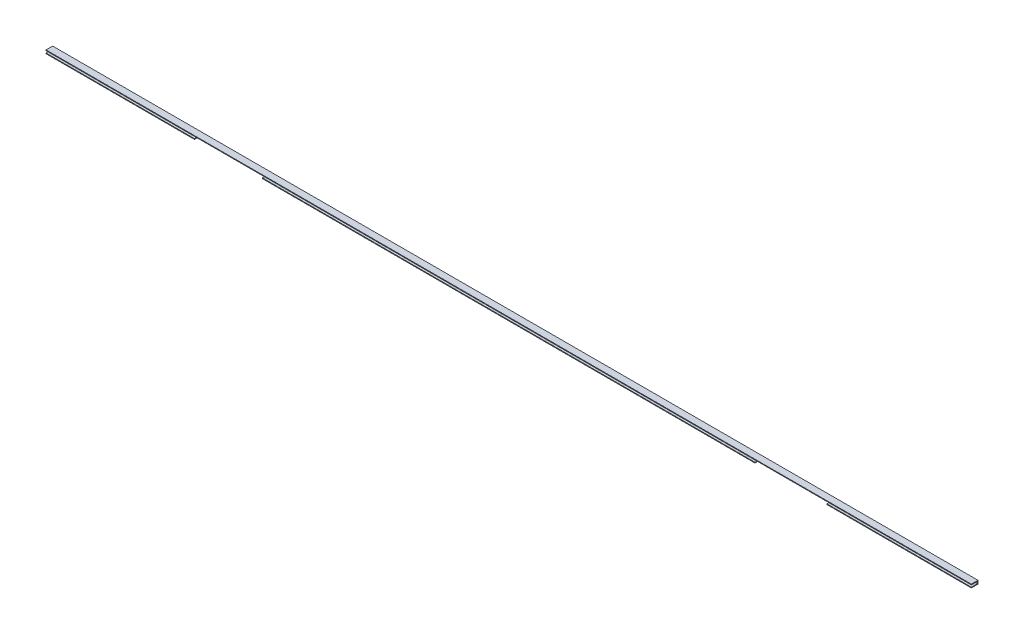
SolidWorks part; units mm, degrees
material "硅橡胶"
ref_plane "前视基准面" through (0, 0, 0) normal (0, 0, 1) x (1, 0, 0)
ref_plane "上视基准面" through (0, 0, 0) normal (0, 1, 0) x (1, 0, 0)
ref_plane "右视基准面" through (0, 0, 0) normal (1, 0, 0) x (0, 0, -1)
other "Configuration Table"
sketch "草图1" plane through (0, 0, 0) normal (0, 0, 1) x (1, 0, 0)
  line L1 (-695, -2.5) -> (695, -2.5)
  line L2 (-695, -2.5) -> (-695, 2.5)
  line L3 (-695, 2.5) -> (695, 2.5)
  line L4 (695, -2.5) -> (695, 2.5)
  line L5 (-695, -2.5) -> (695, 2.5) construction
  line L6 (-695, 2.5) -> (695, -2.5) construction
  point P0 (0, 0)
  dimension "D1" = 1390
  dimension "D2" = 5
extrude "拉伸-薄壁1" add sketch "草图1" along normal blind 10 thin thin type one direction reverse wall 1
sketch "草图2" plane through (-695, 0, 0) normal (-1, 0, 0) x (0, 0, 1)
  line L0 (10, -2.5) -> (0, -2.5) construction
  line L1 (0, 2.5) -> (1, 2.5)
  line L2 (0, 2.5) -> (0, -2.5)
  line L3 (0, -2.5) -> (1, -2.5)
  line L4 (1, 2.5) -> (1, -2.5)
  dimension "D1" = 1
extrude "凸台-拉伸1" add sketch "草图2" against normal up to surface (1389 mm away) contours L4 L3 L2 L1 up to face at (694, 0, 5)
sketch "草图3" plane through (694, 0, 0) normal (-1, 0, 0) x (0, 0, 1)
  line L4 (10, 1.5) -> (1, 1.5)
  line L5 (1, 1.5) -> (1, -1.5)
  line L6 (1, -1.5) -> (10, -1.5)
  line L7 (10, -1.5) -> (10, 1.5)
  line L8 (10, 1.5) -> (1, 1.5)
  line L9 (1, 1.5) -> (1, -1.5)
  line L10 (1, -1.5) -> (10, -1.5)
  line L11 (10, -1.5) -> (10, 1.5)
  dimension "D1" = 0
extrude "切除-拉伸1" cut sketch "草图3" against normal through all both and the other way through all
sketch "草图4" plane through (-695, 0, 0) normal (-1, 0, 0) x (0, 0, 1)
  line L1 (0, -2.5) -> (10, -2.5)
  line L2 (0, -2.5) -> (0, -1.5)
  line L3 (0, -1.5) -> (10, -1.5)
  line L4 (10, -2.5) -> (10, -1.5)
extrude "切除-拉伸2" cut sketch "草图4" along normal blind 102 from offset 325 offset against normal yes
mirror "镜向1" about plane through (0, 0, 0) normal (1, 0, 0) of "切除-拉伸2"
sketch "草图5" plane through (0, -2.5, 0) normal (0, -1, 0) x (1, 0, 0)
  line L0 (472, 10) -> (695, 10) construction
  line L1 (472, 1) -> (478, 1)
  line L2 (472, 1) -> (472, 10)
  line L3 (472, 10) -> (478, 10)
  line L4 (478, 1) -> (478, 10)
  line L6 (472, 1) -> (370, 1) construction
  dimension "D1" = 6
extrude "切除-拉伸5" cut sketch "草图5" against normal up to surface (4 mm away) up to face at (0, 1.5, 5.5)
